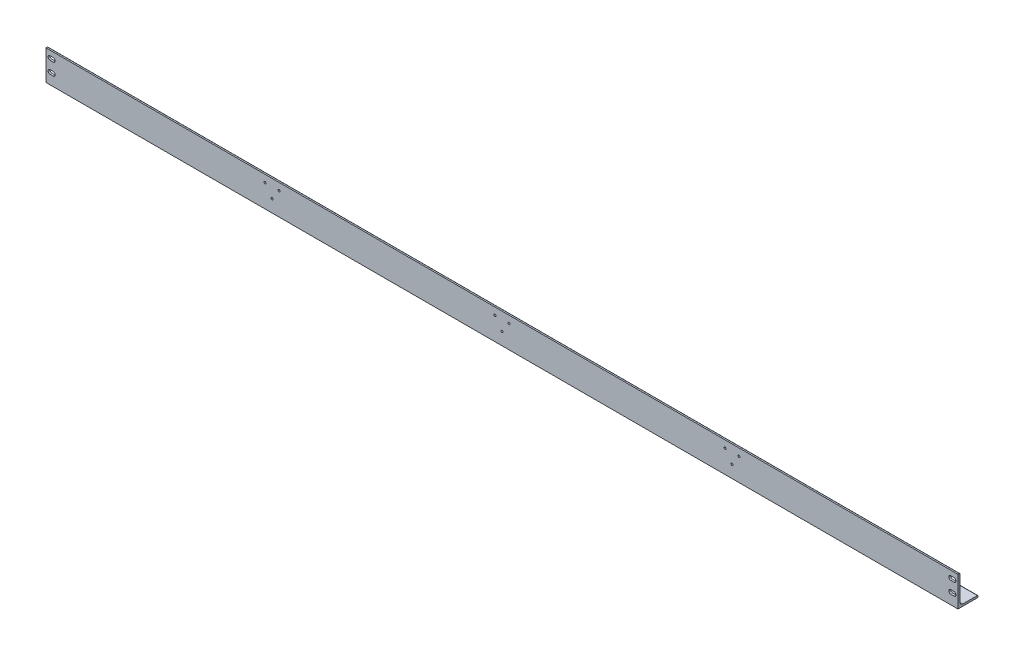
from build123d import *

# Parameters (mm, degrees)
UNEQUAL_ANGLE_7_5_5_5_1_DEPTH = 2276
M6_TAPPED_HOLE2_D             = 5
M6_TAPPED_HOLE2_DEPTH         = 15
M6_TAPPED_HOLE2_TIP           = 1.502151548
M6_TAPPED_HOLE1_D             = 5
M6_TAPPED_HOLE1_DEPTH         = 15
M6_TAPPED_HOLE1_TIP           = 1.502151548
CUT_EXTRUDE1_DEPTH            = 10


with BuildPart() as part:
    # Sketch19 → Unequal angle 7.5-5-5(1) (new body)
    with BuildSketch(Plane.YZ.offset(-1138)):
        with BuildLine():
            Line((75, 0), (0, 0))
            Line((0, 0), (0, -50))
            Line((0, -50), (3.333333333, -50))
            ThreePointArc((3.333333333, -50), (4.511844635, -49.511844635), (5, -48.333333333))
            Line((5, -48.333333333), (5, -13))
            ThreePointArc((5, -13), (7.343145751, -7.343145751), (13, -5))
            Line((13, -5), (73.333333333, -5))
            ThreePointArc((73.333333333, -5), (74.511844635, -4.511844635), (75, -3.333333333))
            Line((75, -3.333333333), (75, 0))
        make_face()
    extrude(amount=UNEQUAL_ANGLE_7_5_5_5_1_DEPTH)

    # M6 Tapped Hole2
    with Locations(Plane(origin=(0, 5, 0), x_dir=(1, 0, 0), z_dir=(0, 1, 0))):
        with Locations((-591.5, 27), (-556.5, 27), (17.5, 27), (-17.5, 27), (591.5, 27), (556.5, 27)):
            Hole(M6_TAPPED_HOLE2_D / 2, depth=M6_TAPPED_HOLE2_DEPTH)
            with Locations((0, 0, -(M6_TAPPED_HOLE2_DEPTH + M6_TAPPED_HOLE2_TIP / 2))):  # 118° drill point
                Cone(0, M6_TAPPED_HOLE2_D / 2, M6_TAPPED_HOLE2_TIP, mode=Mode.SUBTRACT)

    # M6 Tapped Hole1
    with Locations(Plane(origin=(0, 0, -5), x_dir=(-1, 0, 0), z_dir=(0, 0, -1))):
        with Locations((17.5, 56.932613047), (-591.5, 56.932613047), (-556.5, 56.932613047), (-574, 30.932613047), (556.5, 56.932613047), (591.5, 56.932613047), (574, 30.932613047), (-17.5, 56.932613047), (0, 30.932613047)):
            Hole(M6_TAPPED_HOLE1_D / 2, depth=M6_TAPPED_HOLE1_DEPTH)
            with Locations((0, 0, -(M6_TAPPED_HOLE1_DEPTH + M6_TAPPED_HOLE1_TIP / 2))):  # 118° drill point
                Cone(0, M6_TAPPED_HOLE1_D / 2, M6_TAPPED_HOLE1_TIP, mode=Mode.SUBTRACT)

    # Sketch12 → Cut-Extrude1 (cut)
    with BuildSketch(Plane(origin=(0, 0, -5), x_dir=(-1, 0, 0), z_dir=(0, 0, -1))):
        with BuildLine():
            Line((1128, 53), (1120, 53))
            ThreePointArc((1120, 53), (1115, 58), (1120, 63))
            Line((1120, 63), (1128, 63))
            ThreePointArc((1128, 63), (1133, 58), (1128, 53))
        make_face()
        with BuildLine():
            Line((1120, 33), (1128, 33))
            ThreePointArc((1128, 33), (1133, 28), (1128, 23))
            Line((1128, 23), (1120, 23))
            ThreePointArc((1120, 23), (1115, 28), (1120, 33))
        make_face()
        with BuildLine():
            Line((-1128, 63), (-1120, 63))
            ThreePointArc((-1120, 63), (-1115, 58), (-1120, 53))
            Line((-1120, 53), (-1128, 53))
            ThreePointArc((-1128, 53), (-1133, 58), (-1128, 63))
        make_face()
        with BuildLine():
            Line((-1128, 33), (-1120, 33))
            ThreePointArc((-1120, 33), (-1115, 28), (-1120, 23))
            Line((-1120, 23), (-1128, 23))
            ThreePointArc((-1128, 23), (-1133, 28), (-1128, 33))
        make_face()
    extrude(amount=-CUT_EXTRUDE1_DEPTH, mode=Mode.SUBTRACT)


solid = part.part
